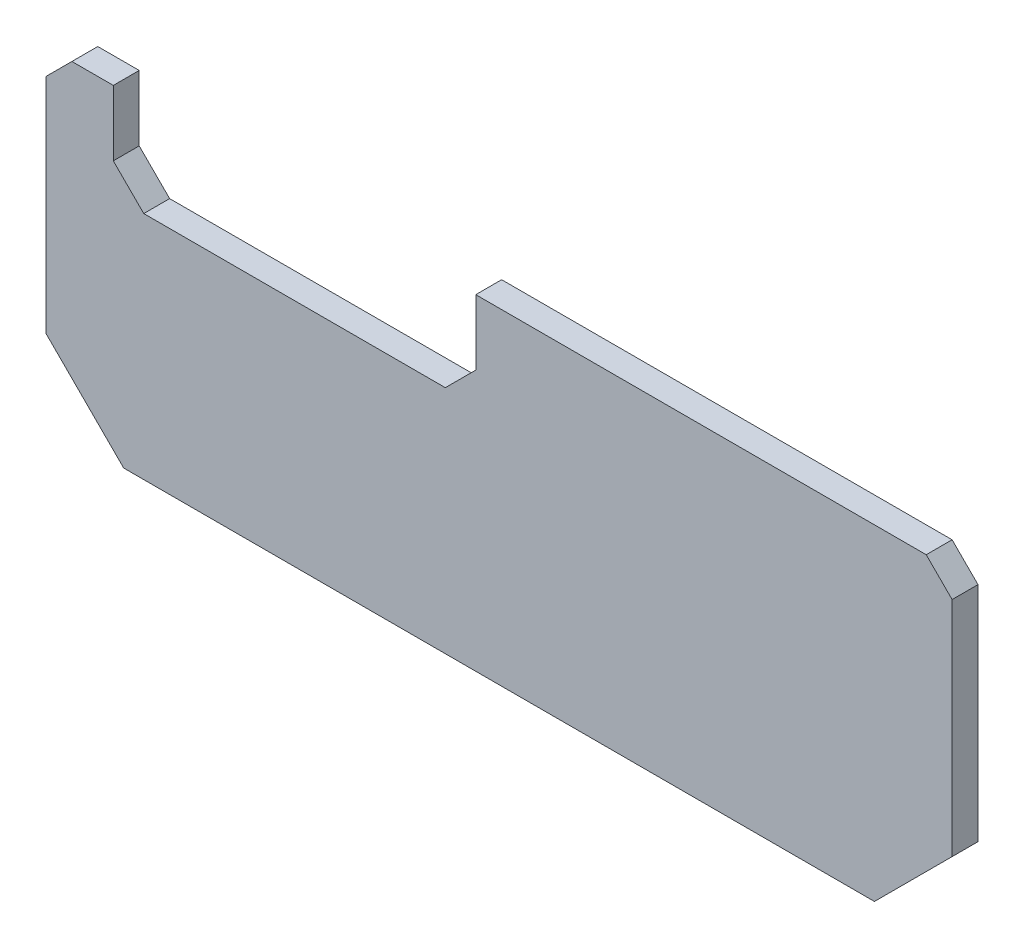
from build123d import *

# Parameters (mm, degrees)
SKETCH1_W           = 175
SKETCH1_H           = 63
BOSS_EXTRUDE1_DEPTH = 5
CUT_EXTRUDE1_DEPTH  = 5
CHAMFER1_SIZE       = 15
CHAMFER2_SIZE       = 5
BOSS_EXTRUDE2_START = -7
BOSS_EXTRUDE2_DEPTH = 25
SKETCH4_W           = 68
SKETCH4_H           = 5
SKETCH4_W_2         = 70
BOSS_EXTRUDE3_DEPTH = 2


with BuildPart() as part:
    # Sketch1 → Boss-Extrude1 (new body)
    with BuildSketch(Plane.XY):
        with Locations((0, 24.5)):
            Rectangle(SKETCH1_W, SKETCH1_H)
    extrude(amount=BOSS_EXTRUDE1_DEPTH)

    # Sketch2 → Cut-Extrude1 (cut)
    with BuildSketch(Plane.XY.offset(5)):
        Polygon((-74.5, 56), (-4.5, 56), (-4.5, 43.378679656), (-10.378679656, 37.5), (-68.621320344, 37.5), (-74.5, 43.378679656), align=None)
    extrude(amount=-CUT_EXTRUDE1_DEPTH, mode=Mode.SUBTRACT)

    # Chamfer1
    chamfer1_edges = [part.edges().sort_by_distance(p)[0] for p in [
        (87.5, -7, 2.5),
        (-87.5, -7, 2.5),
    ]]
    chamfer(chamfer1_edges, length=CHAMFER1_SIZE)

    # Chamfer2
    chamfer2_edges = [part.edges().sort_by_distance(p)[0] for p in [
        (-87.5, 56, 2.5),
        (87.5, 56, 2.5),
    ]]
    chamfer(chamfer2_edges, length=CHAMFER2_SIZE)

    # Sketch3 → Boss-Extrude2 (add)
    with BuildSketch(Plane.XZ.offset(7).offset(BOSS_EXTRUDE2_START)):
        Polygon((51.767949192, 0), (25.232050808, 0), (23.5, -3), (53.5, -3), align=None)
        Polygon((-53.5, -3), (-23.5, -3), (-25.232050808, 0), (-51.767949192, 0), align=None)
    extrude(amount=-BOSS_EXTRUDE2_DEPTH)

    # Sketch4 → Boss-Extrude3 (add)
    with BuildSketch(Plane(origin=(0, 25, 0), x_dir=(1, 0, 0), z_dir=(0, 1, 0))):
        with Locations((-39.5, 2.5)):
            Rectangle(SKETCH4_W, SKETCH4_H)
        with Locations((38.5, 2.5)):
            Rectangle(SKETCH4_W_2, SKETCH4_H)
    extrude(amount=-BOSS_EXTRUDE3_DEPTH)


solid = part.part
